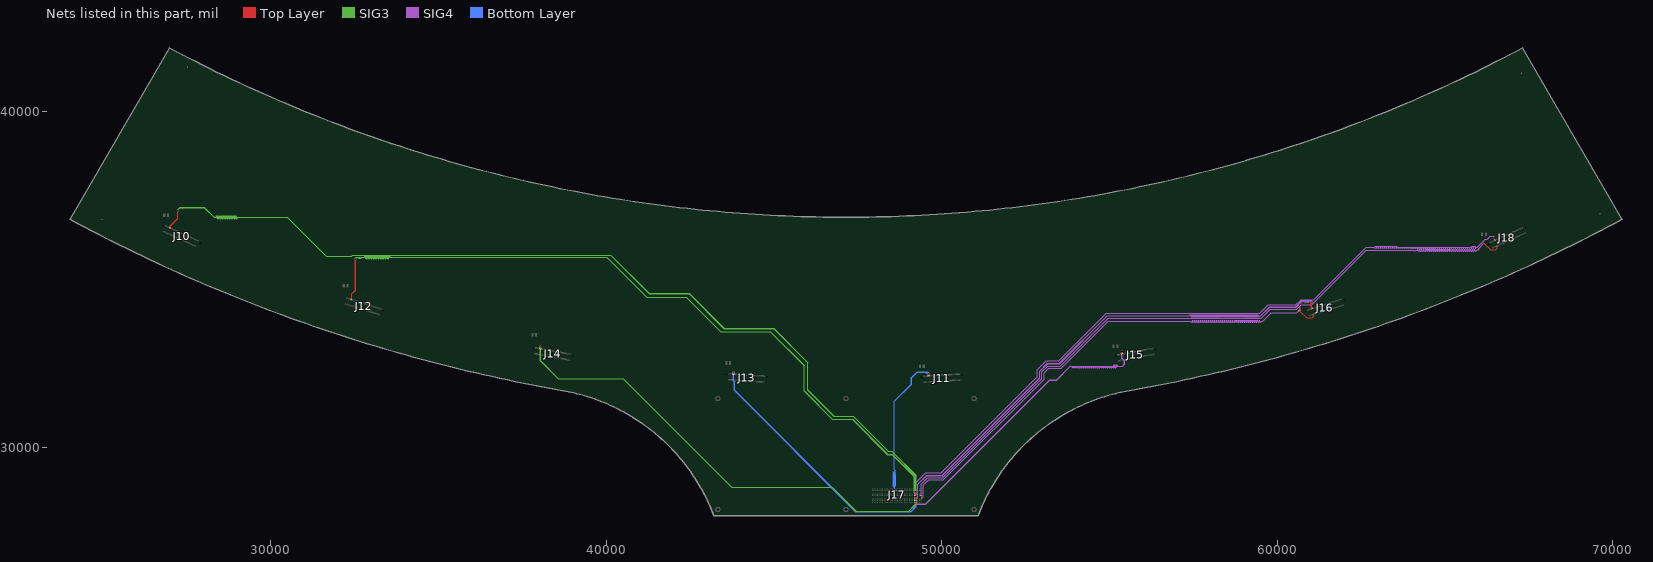
[diagram p0: the nets of this part, all layers, seen from the top]
# Altium PCB MISC86329.PcbDoc (part 2 of 11)
Units mil, origin at the board's own origin, x right, y up, seen from the top; angles counter-clockwise.
Board outline 46247.15 x 13937.21 mil, 6 copper layers (Top Layer, GND2, SIG3, SIG4, POWER5, Bottom Layer); 17 components, 210 nets, 908 pads, 1109 vias.

## Via types
v1: diameter 24, hole 12, Top Layer to Bottom Layer, 684 vias
v2: diameter 18, hole 9, Top Layer to Bottom Layer, 425 vias

## Nets (pads, with @x,y where several pads share a name; then routed paths per layer and width w, separated by ;. In a path a pad name is that pad's centre, name@x,y a point inside that pad or via, vN(x,y) a via of type N, cw(c..) or ccw(c..) an arc to the next point about the centre after c; other vN are vias at no path point) (continued)
CLKP_CH6: J16.9 J17.D1 | length 18297.9
  Top Layer w5: J17.D1@49387.89,28518.8 v2(49411.69,28495) ; v2(60695.5,34183) 60689,34176.5 60689,34050 60873,33866 61037,33866 61087,33916 61087,33946.82 J16.9@61067.89,33965.93
  SIG4 w5: v2(49411.69,28495) 49446,28529.31 49446,28874.86 49608.14,29037 50054.14,29037 53058,32040.86 53058,32231.86 53190.14,32364 53564,32364 54969,33769 57430.43,33769 57435,33764.43 57435,33749.43 57445.43,33739 57464.57,33739 57475,33749.43 57475,33794.43 57479.57,33799 57490.43,33799 57495,33794.43 57495,33749.43 57505.43,33739 57524.57,33739 57535,33749.43 57535,33794.43 57539.57,33799 57550.43,33799 57555,33794.43 57555,33749.43 57565.43,33739 57584.57,33739 57595,33749.43 57595,33794.43 57599.57,33799 57610.43,33799 57615,33794.43 57615,33749.43 57625.43,33739 57644.57,33739 57655,33749.43 57655,33794.43 57659.57,33799 57670.43,33799 57675,33794.43 57675,33749.43 57685.43,33739 57704.57,33739 57715,33749.43 57715,33794.43 57719.57,33799 57730.43,33799 57735,33794.43 57735,33749.43 57745.43,33739 57764.57,33739 57775,33749.43 57775,33794.43 57779.57,33799 57790.43,33799 57795,33794.43 57795,33749.43 57805.43,33739 57824.57,33739 57835,33749.43 57835,33794.43 57839.57,33799 57850.43,33799 57855,33794.43 57855,33749.43 57865.43,33739 57884.57,33739 57895,33749.43 57895,33794.43 57899.57,33799 57910.43,33799 57915,33794.43 57915,33749.43 57925.43,33739 57944.57,33739 57955,33749.43 57955,33794.43 57959.57,33799 57970.43,33799 57975,33794.43 57975,33749.43 57985.43,33739 58004.57,33739 58015,33749.43 58015,33794.43 58019.57,33799 58030.43,33799 58035,33794.43 58035,33749.43 58045.43,33739 58064.57,33739 58075,33749.43 58075,33794.43 58079.57,33799 58090.43,33799 58095,33794.43 58095,33749.43 58105.43,33739 58124.57,33739 58135,33749.43 58135,33794.43 58139.57,33799 58150.43,33799 58155,33794.43 58155,33749.43 58165.43,33739 58184.57,33739 58195,33749.43 58195,33794.43 58199.57,33799 58210.43,33799 58215,33794.43 58215,33749.43 58225.43,33739 58244.57,33739 58255,33749.43 58255,33794.43 58259.57,33799 58270.43,33799 58275,33794.43 58275,33749.43 58285.43,33739 58304.57,33739 58315,33749.43 58315,33794.43 58319.57,33799 58330.43,33799 58335,33794.43 58335,33749.43 58345.43,33739 58364.57,33739 58375,33749.43 58375,33794.43 58379.57,33799 58390.43,33799 58395,33794.43 58395,33749.43 58405.43,33739 58424.57,33739 58435,33749.43 58435,33794.43 58439.57,33799 58450.43,33799 58455,33794.43 58455,33749.43 58465.43,33739 58484.57,33739 58495,33749.43 58495,33794.43 58499.57,33799 58510.43,33799 58515,33794.43 58515,33749.43 58525.43,33739 58544.57,33739 58555,33749.43 58555,33794.43 58559.57,33799 58570.43,33799 58575,33794.43 58575,33749.43 58585.43,33739 58604.57,33739 58615,33749.43 58615,33794.43 58619.57,33799 58630.43,33799 58635,33794.43 58635,33749.43 58645.43,33739 58664.57,33739 58675,33749.43 58675,33794.43 58679.57,33799 58690.43,33799 58695,33794.43 58695,33749.43 58705.43,33739 58724.57,33739 58735,33749.43 58735,33794.43 58739.57,33799 58750.43,33799 58755,33794.43 58755,33749.43 58765.43,33739 58784.57,33739 58795,33749.43 58795,33794.43 58799.57,33799 58810.43,33799 58815,33794.43 58815,33749.43 58825.43,33739 58844.57,33739 58855,33749.43 58855,33794.43 58859.57,33799 58870.43,33799 58875,33794.43 58875,33749.43 58885.43,33739 58904.57,33739 58915,33749.43 58915,33794.43 58919.57,33799 58930.43,33799 58935,33794.43 58935,33749.43 58945.43,33739 58964.57,33739 58975,33749.43 58975,33794.43 58979.57,33799 58990.43,33799 58995,33794.43 58995,33749.43 59005.43,33739 59024.57,33739 59035,33749.43 59035,33794.43 59039.57,33799 59050.43,33799 59055,33794.43 59055,33749.43 59065.43,33739 59084.57,33739 59095,33749.43 59095,33794.43 59099.57,33799 59110.43,33799 59115,33794.43 59115,33749.43 59125.43,33739 59144.57,33739 59155,33749.43 59155,33794.43 59159.57,33799 59170.43,33799 59175,33794.43 59175,33749.43 59185.43,33739 59204.57,33739 59215,33749.43 59215,33794.43 59219.57,33799 59230.43,33799 59235,33794.43 59235,33749.43 59245.43,33739 59264.57,33739 59275,33749.43 59275,33794.43 59279.57,33799 59290.43,33799 59295,33794.43 59295,33749.43 59305.43,33739 59324.57,33739 59335,33749.43 59335,33794.43 59339.57,33799 59350.43,33799 59355,33794.43 59355,33749.43 59365.43,33739 59384.57,33739 59395,33749.43 59395,33794.43 59399.57,33799 59410.43,33799 59415,33794.43 59415,33749.43 59425.43,33739 59444.57,33739 59455,33749.43 59455,33794.43 59459.57,33799 59470.43,33799 59475,33794.43 59475,33749.43 59485.43,33739 59504.57,33739 59515,33749.43 59515,33764.43 59519.57,33769 59564.14,33769 59814.14,34019 60576.14,34019 60622.75,34065.61 60629.82,34065.61 60639.48,34055.95 60646.55,34055.95 60653.62,34063.02 60653.62,34070.09 60643.96,34079.75 60643.96,34086.82 60651.03,34093.89 60658.1,34093.89 60667.76,34084.23 60674.83,34084.23 60681.91,34091.3 60681.91,34098.37 60672.07,34108.21 60672.07,34114.93 60689,34131.86 60689,34175 v2@60696,34182
CLKP_CH7: J17.E1 J18.9 | length 23895.5
  Top Layer w5: J17.E1@49387.89,28568.8 v2(49411.69,28545) ; v2@66159,36106.5 66159,36095 66360,35894 66510,35894 66558,35942 66558,35977.38 J18.9@66532.58,36002.8
  SIG4 w5: v2(49411.69,28545) 49391.69,28565 49391.69,28909.55 49580.14,29098 50036.14,29098 52988,32049.86 52988,32252.86 53159.14,32424 53534.14,32424 54962.14,33852 59519.14,33852 59795.14,34128 60587.14,34128 60719.14,34260 61034.14,34260 62654.14,35880 64053.86,35880 64071.86,35862 64108,35862 64126,35880 64175.57,35880 64186,35890.43 64186,35905.43 64190.57,35910 64201.43,35910 64206,35905.43 64206,35860.43 64216.43,35850 64235.57,35850 64246,35860.43 64246,35905.43 64250.57,35910 64261.43,35910 64266,35905.43 64266,35860.43 64276.43,35850 64295.57,35850 64306,35860.43 64306,35905.43 64310.57,35910 64321.43,35910 64326,35905.43 64326,35860.43 64336.43,35850 64355.57,35850 64366,35860.43 64366,35905.43 64370.57,35910 64381.43,35910 64386,35905.43 64386,35860.43 64396.43,35850 64415.57,35850 64426,35860.43 64426,35905.43 64430.57,35910 64441.43,35910 64446,35905.43 64446,35860.43 64456.43,35850 64475.57,35850 64486,35860.43 64486,35905.43 64490.57,35910 64501.43,35910 64506,35905.43 64506,35860.43 64516.43,35850 64535.57,35850 64546,35860.43 64546,35905.43 64550.57,35910 64561.43,35910 64566,35905.43 64566,35860.43 64576.43,35850 64595.57,35850 64606,35860.43 64606,35905.43 64610.57,35910 64621.43,35910 64626,35905.43 64626,35860.43 64636.43,35850 64655.57,35850 64666,35860.43 64666,35905.43 64670.57,35910 64681.43,35910 64686,35905.43 64686,35860.43 64696.43,35850 64715.57,35850 64726,35860.43 64726,35905.43 64730.57,35910 64741.43,35910 64746,35905.43 64746,35860.43 64756.43,35850 64775.57,35850 64786,35860.43 64786,35905.43 64790.57,35910 64801.43,35910 64806,35905.43 64806,35860.43 64816.43,35850 64835.57,35850 64846,35860.43 64846,35905.43 64850.57,35910 64861.43,35910 64866,35905.43 64866,35860.43 64876.43,35850 64895.57,35850 64906,35860.43 64906,35905.43 64910.57,35910 64921.43,35910 64926,35905.43 64926,35860.43 64936.43,35850 64955.57,35850 64966,35860.43 64966,35905.43 64970.57,35910 64981.43,35910 64986,35905.43 64986,35860.43 64996.43,35850 65015.57,35850 65026,35860.43 65026,35905.43 65030.57,35910 65041.43,35910 65046,35905.43 65046,35860.43 65056.43,35850 65075.57,35850 65086,35860.43 65086,35905.43 65090.57,35910 65101.43,35910 65106,35905.43 65106,35860.43 65116.43,35850 65135.57,35850 65146,35860.43 65146,35905.43 65150.57,35910 65161.43,35910 65166,35905.43 65166,35860.43 65176.43,35850 65195.57,35850 65206,35860.43 65206,35905.43 65210.57,35910 65221.43,35910 65226,35905.43 65226,35860.43 65236.43,35850 65255.57,35850 65266,35860.43 65266,35905.43 65270.57,35910 65281.43,35910 65286,35905.43 65286,35860.43 65296.43,35850 65315.57,35850 65326,35860.43 65326,35905.43 65330.57,35910 65341.43,35910 65346,35905.43 65346,35860.43 65356.43,35850 65375.57,35850 65386,35860.43 65386,35905.43 65390.57,35910 65401.43,35910 65406,35905.43 65406,35860.43 65416.43,35850 65435.57,35850 65446,35860.43 65446,35905.43 65450.57,35910 65461.43,35910 65466,35905.43 65466,35860.43 65476.43,35850 65495.57,35850 65506,35860.43 65506,35905.43 65510.57,35910 65521.43,35910 65526,35905.43 65526,35860.43 65536.43,35850 65555.57,35850 65566,35860.43 65566,35905.43 65570.57,35910 65581.43,35910 65586,35905.43 65586,35860.43 65596.43,35850 65615.57,35850 65626,35860.43 65626,35905.43 65630.57,35910 65641.43,35910 65646,35905.43 65646,35860.43 65656.43,35850 65675.57,35850 65686,35860.43 65686,35905.43 65690.57,35910 65701.43,35910 65706,35905.43 65706,35860.43 65716.43,35850 65735.57,35850 65746,35860.43 65746,35905.43 65750.57,35910 65761.43,35910 65766,35905.43 65766,35860.43 65776.43,35850 65795.57,35850 65806,35860.43 65806,35905.43 65810.57,35910 65821.43,35910 65826,35905.43 65826,35860.43 65836.43,35850 65855.57,35850 65866,35860.43 65866,35905.43 65870.57,35910 65881.43,35910 65886,35905.43 65886,35860.43 65896.43,35850 65915.57,35850 65926,35860.43 65926,35875.43 65930.57,35880 65955.14,35880 65978.32,35903.18 65985.39,35903.18 65994.84,35893.74 66001.91,35893.74 66008.98,35900.81 66008.98,35907.88 65999.54,35917.32 65999.54,35924.39 66159,36083.86 66159,36096 ; 66159,36100 66159,36096 ; v2@66165,36112 66159,36106 66159,36096
  other v2: 66166,36109
DATAIN0N_CH0: J10.12 J17.G5 | length 28226.8
  Top Layer w5: J10.12@27021.23,36536.6 27021.23,36564.2 27024,36566.97 27024,36605.86 27242,36823.86 27242,37050.5 v2(27248.5,37057) ; J17.G5@49187.89,28668.8 v2(49211.69,28692.61)
  SIG3 w5: v2(27248.5,37057) 27242,37063.5 27242,37079.86 27313.14,37151 27337,37151 27352,37151 27357,37146 27357,37136.45 27362,37131.45 27372,37131.45 27377,37136.45 27377,37146 27382,37151 28027.86,37151 28320.86,36858 28375.82,36858 28387.5,36869.68 28387.5,36891.28 28393.32,36897.1 28406.68,36897.1 28412.5,36891.28 28412.5,36830.58 28424.18,36818.9 28445.82,36818.9 28457.5,36830.58 28457.5,36891.28 28463.32,36897.1 28476.68,36897.1 28482.5,36891.28 28482.5,36830.58 28494.18,36818.9 28515.82,36818.9 28527.5,36830.58 28527.5,36891.28 28533.32,36897.1 28546.68,36897.1 28552.5,36891.28 28552.5,36830.58 28564.18,36818.9 28585.82,36818.9 28597.5,36830.58 28597.5,36891.28 28603.32,36897.1 28616.68,36897.1 28622.5,36891.28 28622.5,36830.58 28634.18,36818.9 28655.82,36818.9 28667.5,36830.58 28667.5,36891.28 28673.32,36897.1 28686.68,36897.1 28692.5,36891.28 28692.5,36830.58 28704.18,36818.9 28725.82,36818.9 28737.5,36830.58 28737.5,36891.28 28743.32,36897.1 28756.68,36897.1 28762.5,36891.28 28762.5,36830.58 28774.18,36818.9 28795.82,36818.9 28807.5,36830.58 28807.5,36891.28 28813.32,36897.1 28826.68,36897.1 28832.5,36891.28 28832.5,36830.58 28844.18,36818.9 28865.82,36818.9 28877.5,36830.58 28877.5,36891.28 28883.32,36897.1 28896.68,36897.1 28902.5,36891.28 28902.5,36830.58 28914.18,36818.9 28935.82,36818.9 28947.5,36830.58 28947.5,36891.28 28953.32,36897.1 28966.68,36897.1 28972.5,36891.28 28972.5,36830.58 28984.18,36818.9 29005.82,36818.9 29017.5,36830.58 29017.5,36852.18 29023.32,36858 30497.86,36858 31661.86,35694 32428.14,35694 32459.14,35725 40140.86,35725 41283.86,34582 42471.86,34582 43509.86,33544 44990,33544 46004,32530 46004,31712.86 46790.86,30926 47366.86,30926 48408.86,29884 48514,29884 49231.69,29166.31 49231.69,28712.61 v2(49211.69,28692.61)
DATAIN0N_CH1: J12.12 J17.F5 | length 23094.5
  Top Layer w5: J12.12@32426.41,34405.06 32426.41,34578.41 32536,34688 32536,35605.5 ; J17.F5@49187.89,28618.8 v2(49211.69,28642.61)
  SIG3 w5: v2@32540,35615 32536,35619 32536,35634.86 32565.14,35664 32592,35664 32604.5,35664 32623.25,35664 32629.5,35657.75 32629.5,35642.54 32635.75,35636.29 32648.25,35636.29 32654.5,35642.54 32654.5,35657.75 32660.75,35664 32673.25,35664 32679.5,35657.75 32679.5,35642.54 32685.75,35636.29 32698.25,35636.29 32704.5,35642.54 32704.5,35657.75 32710.75,35664 32791,35664 32809.32,35664 32821,35675.68 32821,35696.87 32826.82,35702.69 32840.18,35702.69 32846,35696.87 32846,35636.99 32857.68,35625.31 32879.32,35625.31 32891,35636.99 32891,35696.87 32896.82,35702.69 32910.18,35702.69 32916,35696.87 32916,35636.99 32927.68,35625.31 32949.32,35625.31 32961,35636.99 32961,35696.87 32966.82,35702.69 32980.18,35702.69 32986,35696.87 32986,35636.99 32997.68,35625.31 33019.32,35625.31 33031,35636.99 33031,35696.87 33036.82,35702.69 33050.18,35702.69 33056,35696.87 33056,35636.99 33067.68,35625.31 33089.32,35625.31 33101,35636.99 33101,35696.87 33106.82,35702.69 33120.18,35702.69 33126,35696.87 33126,35636.99 33137.68,35625.31 33159.32,35625.31 33171,35636.99 33171,35696.87 33176.82,35702.69 33190.18,35702.69 33196,35696.87 33196,35636.99 33207.68,35625.31 33229.32,35625.31 33241,35636.99 33241,35696.87 33246.82,35702.69 33260.18,35702.69 33266,35696.87 33266,35636.99 33277.68,35625.31 33299.32,35625.31 33311,35636.99 33311,35696.87 33316.82,35702.69 33330.18,35702.69 33336,35696.87 33336,35636.99 33347.68,35625.31 33369.32,35625.31 33381,35636.99 33381,35696.87 33386.82,35702.69 33400.18,35702.69 33406,35696.87 33406,35636.99 33417.68,35625.31 33439.32,35625.31 33451,35636.99 33451,35696.87 33456.82,35702.69 33470.18,35702.69 33476,35696.87 33476,35636.99 33487.68,35625.31 33509.32,35625.31 33521,35636.99 33521,35696.87 33526.82,35702.69 33540.18,35702.69 33546,35696.87 33546,35675.68 33557.68,35664 40016.86,35664 41204.86,34476 42383.86,34476 43412.86,33447 44893,33447 45898,32442 45898,31681.86 46741.86,30838 47339.86,30838 48384.86,29793 48524,29793 49181,29136 49181,28675 49203.96,28652.04 49211.69,28644.31 v2(49211.69,28642.61)
  other v2: 32542.5,35612
DATAIN0N_CH2: J14.12 J17.B5 | length 13806
  Top Layer w5: J14.12@38051.07,32948.13 38051.07,32966.93 38045,32973 38045,33024.5 v2(38051.5,33031) ; J17.B5@49187.89,28418.8 v2(49211.69,28395)
  SIG3 w5: v2@38051,33029 38045,33023 38045,32987.14 38052,32980.14 38052,32959.75 38058.25,32953.5 38069.02,32953.5 38075.27,32947.25 38075.27,32934.75 38069.02,32928.5 38058.25,32928.5 38052,32922.25 38052,32586 38580,32058 40518,32058 43751,28825 46736,28825 47451,28110 49021.69,28110 49231.69,28320 49231.69,28375 v2(49211.69,28395)
DATAIN0N_CH3: J13.12 J17.A5 | length 7750
  Top Layer w5: 43800.65,32248.5 43800.65,32225.72 43811.37,32215 J13.12@43811.37,32187.54 ; J17.A5@49187.89,28368.8 v2(49211.69,28345)
  Bottom Layer w5: v2@43810,32255 43807.48,32255 43800,32247.52 43800,32233.75 43806.25,32227.5 43814.53,32227.5 43820.78,32221.25 43820.78,32208.75 43814.53,32202.5 43806.25,32202.5 43800,32196.25 43800,31993 43830,31963 43830,31709 47435,28104 49087.86,28104 49231.69,28247.83 49231.69,28325 v2(49211.69,28345)
  other v2: 43807.15,32255
DATAIN0N_CH4: J11.12 J17.H17 | length 5095.4
  Top Layer w5: v2(48564.09,28742.61) J17.H17@48587.89,28718.8 ; v2(49617.2,32200) 49610.7,32193.5 49610.7,32170.72 49621.42,32160 J11.12@49621.42,32134.62
  Bottom Layer w5: v2(48564.09,28742.61) 48584.09,28762.61 48584.09,28822.43 48579.52,28827 48564.52,28827 48554.09,28837.43 48554.09,28856.57 48564.52,28867 48609.52,28867 48614.09,28871.57 48614.09,28882.43 48609.52,28887 48564.52,28887 48554.09,28897.43 48554.09,28916.57 48564.52,28927 48609.52,28927 48614.09,28931.57 48614.09,28942.43 48609.52,28947 48564.52,28947 48554.09,28957.43 48554.09,28976.57 48564.52,28987 48609.52,28987 48614.09,28991.57 48614.09,29002.43 48609.52,29007 48564.52,29007 48554.09,29017.43 48554.09,29036.57 48564.52,29047 48609.52,29047 48614.09,29051.57 48614.09,29062.43 48609.52,29067 48564.52,29067 48554.09,29077.43 48554.09,29096.57 48564.52,29107 48609.52,29107 48614.09,29111.57 48614.09,29122.43 48609.52,29127 48564.52,29127 48554.09,29137.43 48554.09,29156.57 48564.52,29167 48609.52,29167 48614.09,29171.57 48614.09,29182.43 48609.52,29187 48564.52,29187 48554.09,29197.43 48554.09,29216.57 48564.52,29227 48609.52,29227 48614.09,29231.57 48614.09,29242.43 48609.52,29247 48564.52,29247 48554.09,29257.43 48554.09,29276.57 48564.52,29287 48601.86,29287 48610,29295.14 48610,29307 48584.09,29332.91 48584.09,31378.09 49093,31887 49093,32081 49271,32259 49587.14,32259 49610,32236.14 49610,32209 49616,32203 v2@49616,32201
DATAIN0N_CH5: J15.12 J17.C5 | length 10126.2
  Top Layer w5: J17.C5@49187.89,28468.8 v2(49211.69,28445) ; 55379,32862.5 55379,32831.61 55394.61,32816 J15.12@55394.61,32790.16
  SIG4 w5: v2(49211.69,28445) 49231,28425.69 49231,28336.86 49254.86,28313 49526,28313 53220,32007 53426.14,32007 53837.14,32418 53892.43,32418 53897,32413.43 53897,32388.53 53907.43,32378.1 53926.57,32378.1 53937,32388.53 53937,32413.43 53941.57,32418 53952.43,32418 53957,32413.43 53957,32388.53 53967.43,32378.1 53986.57,32378.1 53997,32388.53 53997,32413.43 54001.57,32418 54012.43,32418 54017,32413.43 54017,32388.53 54027.43,32378.1 54046.57,32378.1 54057,32388.53 54057,32413.43 54061.57,32418 54072.43,32418 54077,32413.43 54077,32388.53 54087.43,32378.1 54106.57,32378.1 54117,32388.53 54117,32413.43 54121.57,32418 54132.43,32418 54137,32413.43 54137,32388.53 54147.43,32378.1 54166.57,32378.1 54177,32388.53 54177,32413.43 54181.57,32418 54192.43,32418 54197,32413.43 54197,32388.53 54207.43,32378.1 54226.57,32378.1 54237,32388.53 54237,32413.43 54241.57,32418 54252.43,32418 54257,32413.43 54257,32388.53 54267.43,32378.1 54286.57,32378.1 54297,32388.53 54297,32413.43 54301.57,32418 54312.43,32418 54317,32413.43 54317,32388.53 54327.43,32378.1 54346.57,32378.1 54357,32388.53 54357,32413.43 54361.57,32418 54372.43,32418 54377,32413.43 54377,32388.53 54387.43,32378.1 54406.57,32378.1 54417,32388.53 54417,32413.43 54421.57,32418 54432.43,32418 54437,32413.43 54437,32388.53 54447.43,32378.1 54466.57,32378.1 54477,32388.53 54477,32413.43 54481.57,32418 54492.43,32418 54497,32413.43 54497,32388.53 54507.43,32378.1 54526.57,32378.1 54537,32388.53 54537,32413.43 54541.57,32418 54552.43,32418 54557,32413.43 54557,32388.53 54567.43,32378.1 54586.57,32378.1 54597,32388.53 54597,32413.43 54601.57,32418 54612.43,32418 54617,32413.43 54617,32388.53 54627.43,32378.1 54646.57,32378.1 54657,32388.53 54657,32413.43 54661.57,32418 54672.43,32418 54677,32413.43 54677,32388.53 54687.43,32378.1 54706.57,32378.1 54717,32388.53 54717,32413.43 54721.57,32418 54732.43,32418 54737,32413.43 54737,32388.53 54747.43,32378.1 54766.57,32378.1 54777,32388.53 54777,32413.43 54781.57,32418 54792.43,32418 54797,32413.43 54797,32388.53 54807.43,32378.1 54826.57,32378.1 54837,32388.53 54837,32413.43 54841.57,32418 54852.43,32418 54857,32413.43 54857,32388.53 54867.43,32378.1 54886.57,32378.1 54897,32388.53 54897,32413.43 54901.57,32418 54912.43,32418 54917,32413.43 54917,32388.53 54927.43,32378.1 54946.57,32378.1 54957,32388.53 54957,32413.43 54961.57,32418 54972.43,32418 54977,32413.43 54977,32388.53 54987.43,32378.1 55006.57,32378.1 55017,32388.53 55017,32413.43 55021.57,32418 55032.43,32418 55037,32413.43 55037,32388.53 55047.43,32378.1 55066.57,32378.1 55077,32388.53 55077,32413.43 55081.57,32418 55092.43,32418 55097,32413.43 55097,32388.53 55107.43,32378.1 55126.57,32378.1 55137,32388.53 55137,32453.33 55141.57,32457.9 55152.43,32457.9 55157,32453.33 55157,32388.53 55167.43,32378.1 55186.57,32378.1 55197,32388.53 55197,32453.33 55201.57,32457.9 55212.43,32457.9 55217,32453.33 55217,32428.43 55227.43,32418 55393.14,32418 55454,32478.86 55454,32588.14 55379,32663.14 55379,32732 55379,32780 55379,32810 55379,32825 55379,32835 55379,32863 v2@55382,32866
  other v2: 55385.5,32869
DATAIN0N_CH6: J16.12 J17.D5 | length 18293.6
  Top Layer w5: J17.D5@49187.89,28518.8 v2(49211.69,28495) ; 61029,34329.5 61029,34160.27 J16.12@61044.87,34144.39
  SIG4 w5: v2(49211.69,28495) 49238.36,28495 49254.86,28511.5 49262.5,28511.5 49282,28531 49282,28906 49549,29173 50016,29173 52916,32073 52916,32280 53150,32514 53509,32514 54930,33935 57387.86,33935 57406.86,33954 57435,33954 57448,33941 57448,33909.57 57452.57,33905 57463.43,33905 57468,33909.57 57468,33954.57 57478.43,33965 57497.57,33965 57508,33954.57 57508,33909.57 57512.57,33905 57523.43,33905 57528,33909.57 57528,33954.57 57538.43,33965 57557.57,33965 57568,33954.57 57568,33909.57 57572.57,33905 57583.43,33905 57588,33909.57 57588,33954.57 57598.43,33965 57617.57,33965 57628,33954.57 57628,33909.57 57632.57,33905 57643.43,33905 57648,33909.57 57648,33954.57 57658.43,33965 57677.57,33965 57688,33954.57 57688,33909.57 57692.57,33905 57703.43,33905 57708,33909.57 57708,33954.57 57718.43,33965 57737.57,33965 57748,33954.57 57748,33909.57 57752.57,33905 57763.43,33905 57768,33909.57 57768,33954.57 57778.43,33965 57797.57,33965 57808,33954.57 57808,33909.57 57812.57,33905 57823.43,33905 57828,33909.57 57828,33954.57 57838.43,33965 57857.57,33965 57868,33954.57 57868,33909.57 57872.57,33905 57883.43,33905 57888,33909.57 57888,33954.57 57898.43,33965 57917.57,33965 57928,33954.57 57928,33909.57 57932.57,33905 57943.43,33905 57948,33909.57 57948,33954.57 57958.43,33965 57977.57,33965 57988,33954.57 57988,33909.57 57992.57,33905 58003.43,33905 58008,33909.57 58008,33954.57 58018.43,33965 58037.57,33965 58048,33954.57 58048,33909.57 58052.57,33905 58063.43,33905 58068,33909.57 58068,33954.57 58078.43,33965 58097.57,33965 58108,33954.57 58108,33909.57 58112.57,33905 58123.43,33905 58128,33909.57 58128,33954.57 58138.43,33965 58157.57,33965 58168,33954.57 58168,33909.57 58172.57,33905 58183.43,33905 58188,33909.57 58188,33954.57 58198.43,33965 58217.57,33965 58228,33954.57 58228,33909.57 58232.57,33905 58243.43,33905 58248,33909.57 58248,33954.57 58258.43,33965 58277.57,33965 58288,33954.57 58288,33909.57 58292.57,33905 58303.43,33905 58308,33909.57 58308,33954.57 58318.43,33965 58337.57,33965 58348,33954.57 58348,33909.57 58352.57,33905 58363.43,33905 58368,33909.57 58368,33954.57 58378.43,33965 58397.57,33965 58408,33954.57 58408,33909.57 58412.57,33905 58423.43,33905 58428,33909.57 58428,33954.57 58438.43,33965 58457.57,33965 58468,33954.57 58468,33909.57 58472.57,33905 58483.43,33905 58488,33909.57 58488,33954.57 58498.43,33965 58517.57,33965 58528,33954.57 58528,33909.57 58532.57,33905 58543.43,33905 58548,33909.57 58548,33954.57 58558.43,33965 58577.57,33965 58588,33954.57 58588,33909.57 58592.57,33905 58603.43,33905 58608,33909.57 58608,33954.57 58618.43,33965 58637.57,33965 58648,33954.57 58648,33909.57 58652.57,33905 58663.43,33905 58668,33909.57 58668,33954.57 58678.43,33965 58697.57,33965 58708,33954.57 58708,33909.57 58712.57,33905 58723.43,33905 58728,33909.57 58728,33954.57 58738.43,33965 58757.57,33965 58768,33954.57 58768,33909.57 58772.57,33905 58783.43,33905 58788,33909.57 58788,33954.57 58798.43,33965 58817.57,33965 58828,33954.57 58828,33909.57 58832.57,33905 58843.43,33905 58848,33909.57 58848,33954.57 58858.43,33965 58877.57,33965 58888,33954.57 58888,33909.57 58892.57,33905 58903.43,33905 58908,33909.57 58908,33954.57 58918.43,33965 58937.57,33965 58948,33954.57 58948,33909.57 58952.57,33905 58963.43,33905 58968,33909.57 58968,33954.57 58978.43,33965 58997.57,33965 59008,33954.57 59008,33909.57 59012.57,33905 59023.43,33905 59028,33909.57 59028,33954.57 59038.43,33965 59057.57,33965 59068,33954.57 59068,33909.57 59072.57,33905 59083.43,33905 59088,33909.57 59088,33954.57 59098.43,33965 59117.57,33965 59128,33954.57 59128,33909.57 59132.57,33905 59143.43,33905 59148,33909.57 59148,33954.57 59158.43,33965 59177.57,33965 59188,33954.57 59188,33909.57 59192.57,33905 59203.43,33905 59208,33909.57 59208,33954.57 59218.43,33965 59237.57,33965 59248,33954.57 59248,33909.57 59252.57,33905 59263.43,33905 59268,33909.57 59268,33954.57 59278.43,33965 59297.57,33965 59308,33954.57 59308,33909.57 59312.57,33905 59323.43,33905 59328,33909.57 59328,33954.57 59338.43,33965 59357.57,33965 59368,33954.57 59368,33909.57 59372.57,33905 59383.43,33905 59388,33909.57 59388,33954.57 59398.43,33965 59417.57,33965 59428,33954.57 59428,33909.57 59432.57,33905 59443.43,33905 59448,33909.57 59448,33924.57 59458.43,33935 59508,33935 59771,34198 60554,34198 60725,34369 61016,34369 61028,34357 61028,34349 ; 61028,34348 61028,34349 ; v2(61035.5,34336) 61035.5,34339.5 61028,34347 61028,34349
DATAIN0N_CH7: J17.E5 J18.12 | length 23896.6
  Top Layer w5: J17.E5@49187.89,28568.8 v2(49211.69,28545) ; 66464,36249.5 66464,36201.11 J18.12@66487.99,36177.13
  SIG4 w5: v2(49211.69,28545) 49231.69,28565 49231.69,28944.69 49530,29243 49988,29243 52850,32105 52850,32314.14 53117.86,32582 53487,32582 54910,34005 59480,34005 59725,34250 60548,34250 60708,34410 61083,34410 62644,35971 62888.57,35971 62899,35960.57 62899,35945.57 62903.57,35941 62914.43,35941 62919,35945.57 62919,35990.57 62929.43,36001 62948.57,36001 62959,35990.57 62959,35945.57 62963.57,35941 62974.43,35941 62979,35945.57 62979,35990.57 62989.43,36001 63008.57,36001 63019,35990.57 63019,35945.57 63023.57,35941 63034.43,35941 63039,35945.57 63039,35990.57 63049.43,36001 63068.57,36001 63079,35990.57 63079,35945.57 63083.57,35941 63094.43,35941 63099,35945.57 63099,35990.57 63109.43,36001 63128.57,36001 63139,35990.57 63139,35945.57 63143.57,35941 63154.43,35941 63159,35945.57 63159,35990.57 63169.43,36001 63188.57,36001 63199,35990.57 63199,35945.57 63203.57,35941 63214.43,35941 63219,35945.57 63219,35990.57 63229.43,36001 63248.57,36001 63259,35990.57 63259,35945.57 63263.57,35941 63274.43,35941 63279,35945.57 63279,35990.57 63289.43,36001 63308.57,36001 63319,35990.57 63319,35945.57 63323.57,35941 63334.43,35941 63339,35945.57 63339,35990.57 63349.43,36001 63368.57,36001 63379,35990.57 63379,35945.57 63383.57,35941 63394.43,35941 63399,35945.57 63399,35990.57 63409.43,36001 63428.57,36001 63439,35990.57 63439,35945.57 63443.57,35941 63454.43,35941 63459,35945.57 63459,35990.57 63469.43,36001 63488.57,36001 63499,35990.57 63499,35945.57 63503.57,35941 63514.43,35941 63519,35945.57 63519,35990.57 63529.43,36001 63548.57,36001 63559,35990.57 63559,35945.57 63563.57,35941 63574.43,35941 63579,35945.57 63579,35960.57 63589.43,35971 63608.57,35971 63619,35960.57 63619,35945.57 63623.57,35941 63634.43,35941 63639,35945.57 63639,35960.57 63649.43,35971 63668.57,35971 63679,35960.57 63679,35945.57 63683.57,35941 63694.43,35941 63699,35945.57 63699,35960.57 63709.43,35971 63728.57,35971 63739,35960.57 63739,35945.57 63743.57,35941 63754.43,35941 63759,35945.57 63759,35960.57 63769.43,35971 63788.57,35971 63799,35960.57 63799,35945.57 63803.57,35941 63814.43,35941 63819,35945.57 63819,35960.57 63829.43,35971 63848.57,35971 63859,35960.57 63859,35945.57 63863.57,35941 63874.43,35941 63879,35945.57 63879,35960.57 63889.43,35971 63908.57,35971 63919,35960.57 63919,35945.57 63923.57,35941 63934.43,35941 63939,35945.57 63939,35960.57 63949.43,35971 63968.57,35971 63979,35960.57 63979,35945.57 63983.57,35941 63994.43,35941 63999,35945.57 63999,35960.57 64009.43,35971 64028.57,35971 64039,35960.57 64039,35945.57 64043.57,35941 64054.43,35941 64059,35945.57 64059,35960.57 64069.43,35971 64088.57,35971 64099,35960.57 64099,35945.57 64103.57,35941 64114.43,35941 64119,35945.57 64119,35960.57 64129.43,35971 64148.57,35971 64159,35960.57 64159,35945.57 64163.57,35941 64174.43,35941 64179,35945.57 64179,35960.57 64189.43,35971 64208.57,35971 64219,35960.57 64219,35945.57 64223.57,35941 64234.43,35941 64239,35945.57 64239,35960.57 64249.43,35971 64268.57,35971 64279,35960.57 64279,35945.57 64283.57,35941 64294.43,35941 64299,35945.57 64299,35960.57 64309.43,35971 64328.57,35971 64339,35960.57 64339,35945.57 64343.57,35941 64354.43,35941 64359,35945.57 64359,35960.57 64369.43,35971 64388.57,35971 64399,35960.57 64399,35945.57 64403.57,35941 64414.43,35941 64419,35945.57 64419,35960.57 64429.43,35971 64448.57,35971 64459,35960.57 64459,35945.57 64463.57,35941 64474.43,35941 64479,35945.57 64479,35960.57 64489.43,35971 64508.57,35971 64519,35960.57 64519,35945.57 64523.57,35941 64534.43,35941 64539,35945.57 64539,35960.57 64549.43,35971 64568.57,35971 64579,35960.57 64579,35945.57 64583.57,35941 64594.43,35941 64599,35945.57 64599,35960.57 64609.43,35971 64628.57,35971 64639,35960.57 64639,35945.57 64643.57,35941 64654.43,35941 64659,35945.57 64659,35960.57 64669.43,35971 64688.57,35971 64699,35960.57 64699,35945.57 64703.57,35941 64714.43,35941 64719,35945.57 64719,35960.57 64729.43,35971 64748.57,35971 64759,35960.57 64759,35945.57 64763.57,35941 64774.43,35941 64779,35945.57 64779,35960.57 64789.43,35971 64808.57,35971 64819,35960.57 64819,35945.57 64823.57,35941 64834.43,35941 64839,35945.57 64839,35960.57 64849.43,35971 64868.57,35971 64879,35960.57 64879,35945.57 64883.57,35941 64894.43,35941 64899,35945.57 64899,35960.57 64909.43,35971 64928.57,35971 64939,35960.57 64939,35945.57 64943.57,35941 64954.43,35941 64959,35945.57 64959,35960.57 64969.43,35971 64988.57,35971 64999,35960.57 64999,35945.57 65003.57,35941 65014.43,35941 65019,35945.57 65019,35960.57 65029.43,35971 65048.57,35971 65059,35960.57 65059,35945.57 65063.57,35941 65074.43,35941 65079,35945.57 65079,35960.57 65089.43,35971 65108.57,35971 65119,35960.57 65119,35945.57 65123.57,35941 65134.43,35941 65139,35945.57 65139,35960.57 65149.43,35971 65168.57,35971 65179,35960.57 65179,35945.57 65183.57,35941 65194.43,35941 65199,35945.57 65199,35960.57 65209.43,35971 65228.57,35971 65239,35960.57 65239,35945.57 65243.57,35941 65254.43,35941 65259,35945.57 65259,35960.57 65269.43,35971 65288.57,35971 65299,35960.57 65299,35945.57 65303.57,35941 65314.43,35941 65319,35945.57 65319,35960.57 65329.43,35971 65348.57,35971 65359,35960.57 65359,35945.57 65363.57,35941 65374.43,35941 65379,35945.57 65379,35960.57 65389.43,35971 65408.57,35971 65419,35960.57 65419,35945.57 65423.57,35941 65434.43,35941 65439,35945.57 65439,35960.57 65449.43,35971 65468.57,35971 65479,35960.57 65479,35945.57 65483.57,35941 65494.43,35941 65499,35945.57 65499,35960.57 65509.43,35971 65528.57,35971 65539,35960.57 65539,35945.57 65543.57,35941 65554.43,35941 65559,35945.57 65559,35960.57 65569.43,35971 65588.57,35971 65599,35960.57 65599,35945.57 65603.57,35941 65614.43,35941 65619,35945.57 65619,35960.57 65629.43,35971 65648.57,35971 65659,35960.57 65659,35945.57 65663.57,35941 65674.43,35941 65679,35945.57 65679,35960.57 65689.43,35971 65708.57,35971 65719,35960.57 65719,35945.57 65723.57,35941 65734.43,35941 65739,35945.57 65739,35960.57 65749.43,35971 65768.57,35971 65779,35960.57 65779,35945.57 65783.57,35941 65794.43,35941 65799,35945.57 65799,35990.57 65809.43,36001 65828.57,36001 65839,35990.57 65839,35945.57 65843.57,35941 65854.43,35941 65859,35945.57 65859,35990.57 65869.43,36001 65888.57,36001 65899,35990.57 65899,35945.57 65903.57,35941 65914.43,35941 65919,35945.57 65919,35960.57 65929.43,35971 65962,35971 66196,36205 66259,36205 66350,36296 66395,36296 66447,36296 66465,36278 66465,36263 v2@66469,36259
  other v2: 66470.5,36256
DATAIN0P_CH0: J10.10 J17.G4 | length 28227.2
  Top Layer w5: J10.10@26992.58,36549.69 27014,36571.11 27014,36610 27232,36828 27232,37050.5 v2(27225.5,37057) ; J17.G4@49237.89,28668.8 v2(49261.69,28692.61)
  SIG3 w5: v2(27225.5,37057) 27232,37063.5 27232,37084 27309,37161 27337,37161 27352,37161 28032,37161 28325,36868 28371.68,36868 28377.5,36873.82 28377.5,36895.42 28389.18,36907.1 28410.82,36907.1 28422.5,36895.42 28422.5,36834.72 28428.32,36828.9 28441.68,36828.9 28447.5,36834.72 28447.5,36895.42 28459.18,36907.1 28480.82,36907.1 28492.5,36895.42 28492.5,36834.72 28498.32,36828.9 28511.68,36828.9 28517.5,36834.72 28517.5,36895.42 28529.18,36907.1 28550.82,36907.1 28562.5,36895.42 28562.5,36834.72 28568.32,36828.9 28581.68,36828.9 28587.5,36834.72 28587.5,36895.42 28599.18,36907.1 28620.82,36907.1 28632.5,36895.42 28632.5,36834.72 28638.32,36828.9 28651.68,36828.9 28657.5,36834.72 28657.5,36895.42 28669.18,36907.1 28690.82,36907.1 28702.5,36895.42 28702.5,36834.72 28708.32,36828.9 28721.68,36828.9 28727.5,36834.72 28727.5,36895.42 28739.18,36907.1 28760.82,36907.1 28772.5,36895.42 28772.5,36834.72 28778.32,36828.9 28791.68,36828.9 28797.5,36834.72 28797.5,36895.42 28809.18,36907.1 28830.82,36907.1 28842.5,36895.42 28842.5,36834.72 28848.32,36828.9 28861.68,36828.9 28867.5,36834.72 28867.5,36895.42 28879.18,36907.1 28900.82,36907.1 28912.5,36895.42 28912.5,36834.72 28918.32,36828.9 28931.68,36828.9 28937.5,36834.72 28937.5,36895.42 28949.18,36907.1 28970.82,36907.1 28982.5,36895.42 28982.5,36834.72 28988.32,36828.9 29001.68,36828.9 29007.5,36834.72 29007.5,36856.32 29019.18,36868 30502,36868 31666,35704 32424,35704 32455,35735 40145,35735 41288,34592 42476,34592 43514,33554 44994.14,33554 46014,32534.14 46014,31717 46795,30936 47371,30936 48413,29894 48518.14,29894 49241.69,29170.45 49241.69,28712.61 v2(49261.69,28692.61)
DATAIN0P_CH1: J12.10 J17.F4 | length 23095.5
  Top Layer w5: J12.10@32396.38,34414.57 32415,34433.18 32415,34581.14 32526,34692.14 32526,35605.5 v2(32519.5,35612) ; J17.F4@49237.89,28618.8 v2(49261.69,28642.61)
  SIG3 w5: v2@32520,35614 32526,35620 32526,35629 ; 32526,35626 32526,35629 ; v2(49261.69,28642.61) 49235.03,28642.61 49218.53,28659.11 49211.04,28659.11 49191,28679.14 49191,29140.14 48528.14,29803 48389,29803 47344,30848 46746,30848 45908,31686 45908,32446.14 44897.14,33457 43417,33457 42388,34486 41209,34486 40021,35674 33561.82,35674 33556,35679.82 33556,35701.01 33544.32,35712.69 33522.68,35712.69 33511,35701.01 33511,35641.13 33505.18,35635.31 33491.82,35635.31 33486,35641.13 33486,35701.01 33474.32,35712.69 33452.68,35712.69 33441,35701.01 33441,35641.13 33435.18,35635.31 33421.82,35635.31 33416,35641.13 33416,35701.01 33404.32,35712.69 33382.68,35712.69 33371,35701.01 33371,35641.13 33365.18,35635.31 33351.82,35635.31 33346,35641.13 33346,35701.01 33334.32,35712.69 33312.68,35712.69 33301,35701.01 33301,35641.13 33295.18,35635.31 33281.82,35635.31 33276,35641.13 33276,35701.01 33264.32,35712.69 33242.68,35712.69 33231,35701.01 33231,35641.13 33225.18,35635.31 33211.82,35635.31 33206,35641.13 33206,35701.01 33194.32,35712.69 33172.68,35712.69 33161,35701.01 33161,35641.13 33155.18,35635.31 33141.82,35635.31 33136,35641.13 33136,35701.01 33124.32,35712.69 33102.68,35712.69 33091,35701.01 33091,35641.13 33085.18,35635.31 33071.82,35635.31 33066,35641.13 33066,35701.01 33054.32,35712.69 33032.68,35712.69 33021,35701.01 33021,35641.13 33015.18,35635.31 33001.82,35635.31 32996,35641.13 32996,35701.01 32984.32,35712.69 32962.68,35712.69 32951,35701.01 32951,35641.13 32945.18,35635.31 32931.82,35635.31 32926,35641.13 32926,35701.01 32914.32,35712.69 32892.68,35712.69 32881,35701.01 32881,35641.13 32875.18,35635.31 32861.82,35635.31 32856,35641.13 32856,35701.01 32844.32,35712.69 32822.68,35712.69 32811,35701.01 32811,35679.82 32805.18,35674 32791,35674 32710.75,35674 32673.25,35674 32660.75,35674 32623.25,35674 32604.5,35674 32592,35674 32561,35674 32526,35639 32526,35629
DATAIN0P_CH2: J14.10 J17.B4 | length 13806.5
  Top Layer w5: J14.10@38020.11,32953.91 38020.11,32963.11 38035,32978 38035,33024.5 v2(38028.5,33031) ; J17.B4@49237.89,28418.8 v2(49261.69,28395)
  SIG3 w5: v2@38028,33030 38035,33023 38035,32983 38042,32976 38042,32959.75 38042,32581.86 38575.86,32048 40513.86,32048 43746.86,28815 46731.86,28815 47446.86,28100 49025.83,28100 49241.69,28315.86 49241.69,28375 v2(49261.69,28395)
DATAIN0P_CH3: J13.10 J17.A4 | length 7750.7
  Top Layer w5: J13.10@43779.93,32189.5 43779.93,32215 43790.65,32225.72 43790.65,32248.5 ; J17.A4@49237.89,28368.8 v2(49261.69,28345)
  Bottom Layer w5: v2@43785,32255 43790,32250 43790,32233.75 43790,31988.86 43820,31958.86 43820,31704.86 47430.86,28094 49092,28094 49241.69,28243.69 49241.69,28325 v2(49261.69,28345)
  other v2: 43784.15,32255
DATAIN0P_CH4: J11.10 J17.H16 | length 5095
  Top Layer w5: v2(48614.09,28742.61) J17.H16@48637.89,28718.8 ; J11.10@49589.98,32132.74 49589.98,32158 49600.7,32168.72 49600.7,32193.5
  Bottom Layer w5: v2(48614.09,28742.61) 48594.09,28762.61 48594.09,28826.57 48583.66,28837 48568.66,28837 48564.09,28841.57 48564.09,28852.43 48568.66,28857 48613.66,28857 48624.09,28867.43 48624.09,28886.57 48613.66,28897 48568.66,28897 48564.09,28901.57 48564.09,28912.43 48568.66,28917 48613.66,28917 48624.09,28927.43 48624.09,28946.57 48613.66,28957 48568.66,28957 48564.09,28961.57 48564.09,28972.43 48568.66,28977 48613.66,28977 48624.09,28987.43 48624.09,29006.57 48613.66,29017 48568.66,29017 48564.09,29021.57 48564.09,29032.43 48568.66,29037 48613.66,29037 48624.09,29047.43 48624.09,29066.57 48613.66,29077 48568.66,29077 48564.09,29081.57 48564.09,29092.43 48568.66,29097 48613.66,29097 48624.09,29107.43 48624.09,29126.57 48613.66,29137 48568.66,29137 48564.09,29141.57 48564.09,29152.43 48568.66,29157 48613.66,29157 48624.09,29167.43 48624.09,29186.57 48613.66,29197 48568.66,29197 48564.09,29201.57 48564.09,29212.43 48568.66,29217 48613.66,29217 48624.09,29227.43 48624.09,29246.57 48613.66,29257 48568.66,29257 48564.09,29261.57 48564.09,29272.43 48568.66,29277 48606,29277 48620,29291 48620,29311.14 48594.09,29337.06 48594.09,31373.94 49103,31882.86 49103,32076.86 49275.14,32249 49524,32249 49529,32244 49529,32226.24 49534,32221.24 49544,32221.24 49549,32226.24 49549,32244 49554,32249 49583,32249 49600,32232 49600,32208 v2@49596,32204
  other v2: 49594.2,32200
DATAIN0P_CH5: J15.10 J17.C4 | length 10125.8
  Top Layer w5: J17.C4@49237.89,28468.8 v2(49261.69,28445) ; J15.10@55363.63,32784.46 55363.63,32811 55369,32816.37 55369,32862.5
  SIG4 w5: v2(49261.69,28445) 49241,28424.31 49241,28341 49259,28323 49521.86,28323 53215.86,32017 53422,32017 53833,32428 53896.57,32428 53907,32417.57 53907,32392.67 53911.57,32388.1 53922.43,32388.1 53927,32392.67 53927,32417.57 53937.43,32428 53956.57,32428 53967,32417.57 53967,32392.67 53971.57,32388.1 53982.43,32388.1 53987,32392.67 53987,32417.57 53997.43,32428 54016.57,32428 54027,32417.57 54027,32392.67 54031.57,32388.1 54042.43,32388.1 54047,32392.67 54047,32417.57 54057.43,32428 54076.57,32428 54087,32417.57 54087,32392.67 54091.57,32388.1 54102.43,32388.1 54107,32392.67 54107,32417.57 54117.43,32428 54136.57,32428 54147,32417.57 54147,32392.67 54151.57,32388.1 54162.43,32388.1 54167,32392.67 54167,32417.57 54177.43,32428 54196.57,32428 54207,32417.57 54207,32392.67 54211.57,32388.1 54222.43,32388.1 54227,32392.67 54227,32417.57 54237.43,32428 54256.57,32428 54267,32417.57 54267,32392.67 54271.57,32388.1 54282.43,32388.1 54287,32392.67 54287,32417.57 54297.43,32428 54316.57,32428 54327,32417.57 54327,32392.67 54331.57,32388.1 54342.43,32388.1 54347,32392.67 54347,32417.57 54357.43,32428 54376.57,32428 54387,32417.57 54387,32392.67 54391.57,32388.1 54402.43,32388.1 54407,32392.67 54407,32417.57 54417.43,32428 54436.57,32428 54447,32417.57 54447,32392.67 54451.57,32388.1 54462.43,32388.1 54467,32392.67 54467,32417.57 54477.43,32428 54496.57,32428 54507,32417.57 54507,32392.67 54511.57,32388.1 54522.43,32388.1 54527,32392.67 54527,32417.57 54537.43,32428 54556.57,32428 54567,32417.57 54567,32392.67 54571.57,32388.1 54582.43,32388.1 54587,32392.67 54587,32417.57 54597.43,32428 54616.57,32428 54627,32417.57 54627,32392.67 54631.57,32388.1 54642.43,32388.1 54647,32392.67 54647,32417.57 54657.43,32428 54676.57,32428 54687,32417.57 54687,32392.67 54691.57,32388.1 54702.43,32388.1 54707,32392.67 54707,32417.57 54717.43,32428 54736.57,32428 54747,32417.57 54747,32392.67 54751.57,32388.1 54762.43,32388.1 54767,32392.67 54767,32417.57 54777.43,32428 54796.57,32428 54807,32417.57 54807,32392.67 54811.57,32388.1 54822.43,32388.1 54827,32392.67 54827,32417.57 54837.43,32428 54856.57,32428 54867,32417.57 54867,32392.67 54871.57,32388.1 54882.43,32388.1 54887,32392.67 54887,32417.57 54897.43,32428 54916.57,32428 54927,32417.57 54927,32392.67 54931.57,32388.1 54942.43,32388.1 54947,32392.67 54947,32417.57 54957.43,32428 54976.57,32428 54987,32417.57 54987,32392.67 54991.57,32388.1 55002.43,32388.1 55007,32392.67 55007,32417.57 55017.43,32428 55036.57,32428 55047,32417.57 55047,32392.67 55051.57,32388.1 55062.43,32388.1 55067,32392.67 55067,32417.57 55077.43,32428 55096.57,32428 55107,32417.57 55107,32392.67 55111.57,32388.1 55122.43,32388.1 55127,32392.67 55127,32457.47 55137.43,32467.9 55156.57,32467.9 55167,32457.47 55167,32392.67 55171.57,32388.1 55182.43,32388.1 55187,32392.67 55187,32457.47 55197.43,32467.9 55216.57,32467.9 55227,32457.47 55227,32432.57 55231.57,32428 55389,32428 55444,32483 55444,32584 55369,32659 55369,32732 55369,32780 55364,32785 55352.84,32785 55347.84,32790 55347.84,32800 55352.84,32805 55364,32805 55369,32810 55369,32825 55369,32835 55369,32863 v2@55366,32866
  other v2: 55362.5,32869
DATAIN0P_CH6: J16.10 J17.D4 | length 18292.9
  Top Layer w5: J17.D4@49237.89,28518.8 v2(49261.69,28495) ; J16.10@61014.82,34134.96 61014.82,34162 61019,34166.18 61019,34329.5
  SIG4 w5: v2(49261.69,28495) 49292,28525.31 49292,28901.86 49553.14,29163 50020.14,29163 52926,32068.86 52926,32275.86 53154.14,32504 53513.14,32504 54934.14,33925 57392,33925 57411,33944 57430.86,33944 57438,33936.86 57438,33905.43 57448.43,33895 57467.57,33895 57478,33905.43 57478,33950.43 57482.57,33955 57493.43,33955 57498,33950.43 57498,33905.43 57508.43,33895 57527.57,33895 57538,33905.43 57538,33950.43 57542.57,33955 57553.43,33955 57558,33950.43 57558,33905.43 57568.43,33895 57587.57,33895 57598,33905.43 57598,33950.43 57602.57,33955 57613.43,33955 57618,33950.43 57618,33905.43 57628.43,33895 57647.57,33895 57658,33905.43 57658,33950.43 57662.57,33955 57673.43,33955 57678,33950.43 57678,33905.43 57688.43,33895 57707.57,33895 57718,33905.43 57718,33950.43 57722.57,33955 57733.43,33955 57738,33950.43 57738,33905.43 57748.43,33895 57767.57,33895 57778,33905.43 57778,33950.43 57782.57,33955 57793.43,33955 57798,33950.43 57798,33905.43 57808.43,33895 57827.57,33895 57838,33905.43 57838,33950.43 57842.57,33955 57853.43,33955 57858,33950.43 57858,33905.43 57868.43,33895 57887.57,33895 57898,33905.43 57898,33950.43 57902.57,33955 57913.43,33955 57918,33950.43 57918,33905.43 57928.43,33895 57947.57,33895 57958,33905.43 57958,33950.43 57962.57,33955 57973.43,33955 57978,33950.43 57978,33905.43 57988.43,33895 58007.57,33895 58018,33905.43 58018,33950.43 58022.57,33955 58033.43,33955 58038,33950.43 58038,33905.43 58048.43,33895 58067.57,33895 58078,33905.43 58078,33950.43 58082.57,33955 58093.43,33955 58098,33950.43 58098,33905.43 58108.43,33895 58127.57,33895 58138,33905.43 58138,33950.43 58142.57,33955 58153.43,33955 58158,33950.43 58158,33905.43 58168.43,33895 58187.57,33895 58198,33905.43 58198,33950.43 58202.57,33955 58213.43,33955 58218,33950.43 58218,33905.43 58228.43,33895 58247.57,33895 58258,33905.43 58258,33950.43 58262.57,33955 58273.43,33955 58278,33950.43 58278,33905.43 58288.43,33895 58307.57,33895 58318,33905.43 58318,33950.43 58322.57,33955 58333.43,33955 58338,33950.43 58338,33905.43 58348.43,33895 58367.57,33895 58378,33905.43 58378,33950.43 58382.57,33955 58393.43,33955 58398,33950.43 58398,33905.43 58408.43,33895 58427.57,33895 58438,33905.43 58438,33950.43 58442.57,33955 58453.43,33955 58458,33950.43 58458,33905.43 58468.43,33895 58487.57,33895 58498,33905.43 58498,33950.43 58502.57,33955 58513.43,33955 58518,33950.43 58518,33905.43 58528.43,33895 58547.57,33895 58558,33905.43 58558,33950.43 58562.57,33955 58573.43,33955 58578,33950.43 58578,33905.43 58588.43,33895 58607.57,33895 58618,33905.43 58618,33950.43 58622.57,33955 58633.43,33955 58638,33950.43 58638,33905.43 58648.43,33895 58667.57,33895 58678,33905.43 58678,33950.43 58682.57,33955 58693.43,33955 58698,33950.43 58698,33905.43 58708.43,33895 58727.57,33895 58738,33905.43 58738,33950.43 58742.57,33955 58753.43,33955 58758,33950.43 58758,33905.43 58768.43,33895 58787.57,33895 58798,33905.43 58798,33950.43 58802.57,33955 58813.43,33955 58818,33950.43 58818,33905.43 58828.43,33895 58847.57,33895 58858,33905.43 58858,33950.43 58862.57,33955 58873.43,33955 58878,33950.43 58878,33905.43 58888.43,33895 58907.57,33895 58918,33905.43 58918,33950.43 58922.57,33955 58933.43,33955 58938,33950.43 58938,33905.43 58948.43,33895 58967.57,33895 58978,33905.43 58978,33950.43 58982.57,33955 58993.43,33955 58998,33950.43 58998,33905.43 59008.43,33895 59027.57,33895 59038,33905.43 59038,33950.43 59042.57,33955 59053.43,33955 59058,33950.43 59058,33905.43 59068.43,33895 59087.57,33895 59098,33905.43 59098,33950.43 59102.57,33955 59113.43,33955 59118,33950.43 59118,33905.43 59128.43,33895 59147.57,33895 59158,33905.43 59158,33950.43 59162.57,33955 59173.43,33955 59178,33950.43 59178,33905.43 59188.43,33895 59207.57,33895 59218,33905.43 59218,33950.43 59222.57,33955 59233.43,33955 59238,33950.43 59238,33905.43 59248.43,33895 59267.57,33895 59278,33905.43 59278,33950.43 59282.57,33955 59293.43,33955 59298,33950.43 59298,33905.43 59308.43,33895 59327.57,33895 59338,33905.43 59338,33950.43 59342.57,33955 59353.43,33955 59358,33950.43 59358,33905.43 59368.43,33895 59387.57,33895 59398,33905.43 59398,33950.43 59402.57,33955 59413.43,33955 59418,33950.43 59418,33905.43 59428.43,33895 59447.57,33895 59458,33905.43 59458,33920.43 59462.57,33925 59512.14,33925 59775.14,34188 60558.14,34188 60729.14,34359 60879,34359 60884,34354 60884,34340.66 60889,34335.66 60899,34335.66 60904,34340.66 60904,34354 60909,34359 60919,34359 60924,34354 60924,34340.66 60929,34335.66 60939,34335.66 60944,34340.66 60944,34354 60949,34359 61011.86,34359 61018,34352.86 61018,34343 v2@61014,34339
  other v2: 61012.5,34336